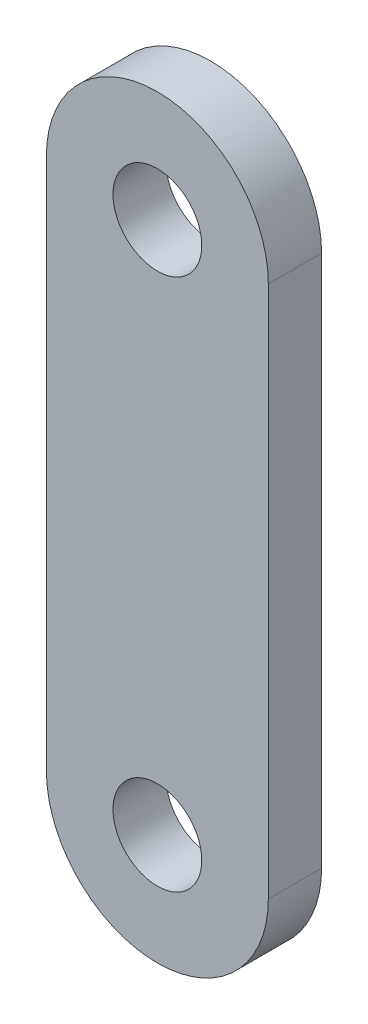
from build123d import *

# Parameters (mm, degrees)
SKETCH1_R           = 5
BOSS_EXTRUDE1_DEPTH = 3


with BuildPart() as part:
    # Sketch1 → Boss-Extrude1 (new, symmetric)
    with BuildSketch(Plane.XY):
        with BuildLine():
            Line((-12.5, 0), (-12.5, 60))
            ThreePointArc((-12.5, 60), (0, 72.5), (12.5, 60))
            Line((12.5, 60), (12.5, 0))
            ThreePointArc((12.5, 0), (0, -12.5), (-12.5, 0))
        make_face()
        Circle(SKETCH1_R, mode=Mode.SUBTRACT)
        with Locations((0, 60)):
            Circle(SKETCH1_R, mode=Mode.SUBTRACT)
    extrude(amount=BOSS_EXTRUDE1_DEPTH, both=True)


solid = part.part
